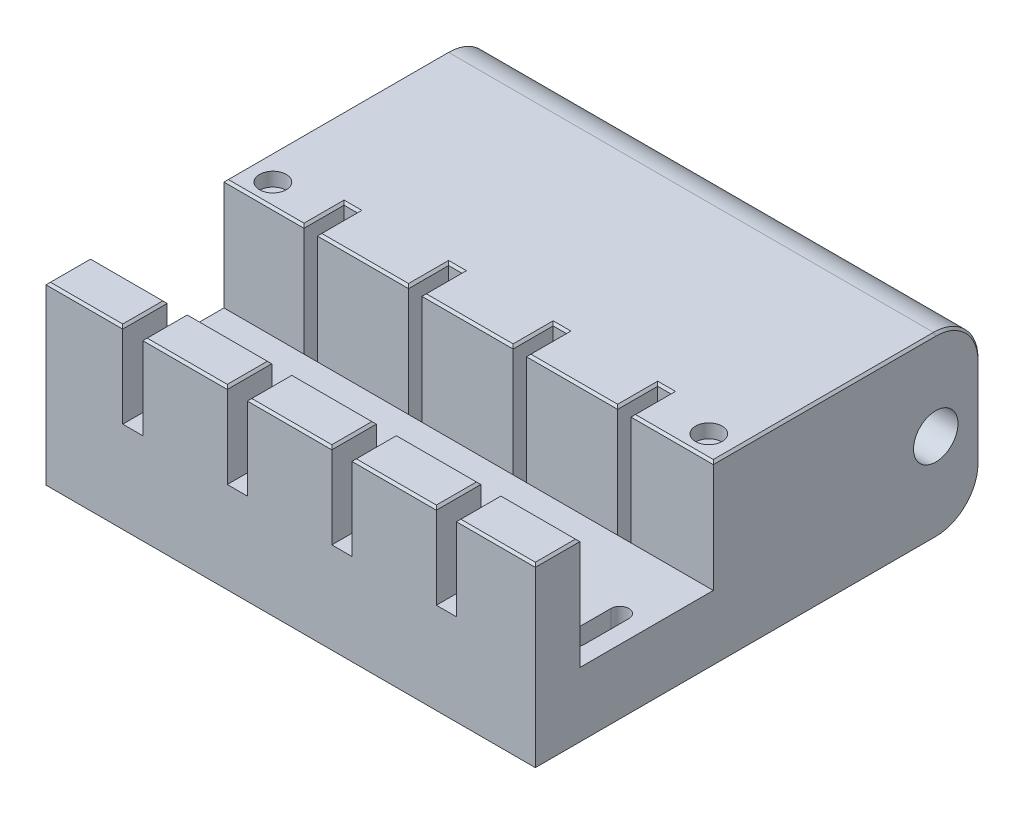
SolidWorks part; units mm, degrees
ref_plane "Front Plane" through (0, 0, 0) normal (0, 0, 1) x (1, 0, 0)
ref_plane "Top Plane" through (0, 0, 0) normal (0, 1, 0) x (1, 0, 0)
ref_plane "Right Plane" through (0, 0, 0) normal (1, 0, 0) x (0, 0, -1)
other "Configuration Table"
sketch "Sketch7" plane through (0, 0, 0) normal (0, 1, 0) x (1, 0, 0)
  line L1 (-55, 50) -> (55, 50)
  line L2 (-55, 50) -> (-55, -50)
  line L3 (-55, -50) -> (55, -50)
  line L4 (55, 50) -> (55, -50)
  line L5 (-55, 50) -> (55, -50) construction
  line L6 (-55, -50) -> (55, 50) construction
  point P0 (0, 0)
  dimension "D1" = 110
  dimension "D2" = 100
extrude "Boss-Extrude2" add sketch "Sketch7" along normal blind 40
sketch "Sketch8" plane through (0, 40, 0) normal (0, 1, 0) x (1, 0, 0)
  line L0 (0, 50) -> (0, -50) construction
  line L1 (55, 50) -> (-55, 50) construction
  line L2 (-55, -50) -> (55, -50) construction
  line L3 (-55, 50) -> (-55, -50) construction
  line L4 (-37, -1) -> (-34, -1)
  line L5 (-37, -1) -> (-37, -10)
  line L6 (-37, -10) -> (-34, -10)
  line L7 (-34, -1) -> (-34, -10)
  line L8 (-37, -1) -> (-34, -10) construction
  line L9 (-37, -10) -> (-34, -1) construction
  line L10 (-13.5, -1) -> (-13.5, -10)
  line L11 (-13.5, -1) -> (-10.5, -1)
  line L12 (-10.5, -1) -> (-10.5, -10)
  line L13 (-13.5, -10) -> (-10.5, -10)
  line L14 (10, -1) -> (10, -10)
  line L15 (10, -1) -> (13, -1)
  line L16 (13, -1) -> (13, -10)
  line L17 (10, -10) -> (13, -10)
  line L18 (33.5, -1) -> (33.5, -10)
  line L19 (33.5, -10) -> (36.5, -10)
  line L20 (36.5, -1) -> (36.5, -10)
  line L21 (33.5, -1) -> (36.5, -1)
  point P6 (-35.5, -5.5)
  dimension "D1" = 3
  dimension "D2" = 9
  dimension "D3" = 40
  dimension "D4" = 18
  dimension "D6" = 20.5
  dimension "D8" = 23.5
  dimension "D5" = 3
  dimension "D7" = 2
extrude "Cut-Extrude1" cut sketch "Sketch8" against normal through all
sketch "Sketch9" plane through (55, 0, 0) normal (1, 0, 0) x (0, 0, -1)
  line L0 (-40, 15) -> (-40, 40)
  line L2 (-50, 40) -> (50, 40) construction
  line L3 (-40, 15) -> (-10, 15)
  line L4 (-40, 40) -> (-10, 40)
  line L5 (-10, 40) -> (-10, 15)
  line L6 (-50, 40) -> (-50, 0) construction
  dimension "D1" = 25
  dimension "D2" = 10
  dimension "D4" = 30
sketch "Sketch11" plane through (0, 40, 0) normal (0, 1, 0) x (1, 0, 0)
  line L0 (-37, -10) -> (-34, -10) construction
  line L1 (-37.75, -35) -> (-33.25, -35)
  line L2 (-37.75, -35) -> (-37.75, -52)
  line L3 (-37.75, -52) -> (-33.25, -52)
  line L4 (-33.25, -35) -> (-33.25, -52)
  line L5 (-55, -50) -> (55, -50) construction
  line L6 (-14.25, -35) -> (-14.25, -52)
  line L7 (-14.25, -35) -> (-9.75, -35)
  line L8 (-9.75, -35) -> (-9.75, -52)
  line L9 (-14.25, -52) -> (-9.75, -52)
  line L10 (9.25, -35) -> (9.25, -52)
  line L11 (9.25, -35) -> (13.75, -35)
  line L12 (13.75, -35) -> (13.75, -52)
  line L13 (9.25, -52) -> (13.75, -52)
  line L14 (32.75, -35) -> (32.75, -52)
  line L15 (32.75, -35) -> (37.25, -35)
  line L16 (37.25, -35) -> (37.25, -52)
  line L17 (32.75, -52) -> (37.25, -52)
  point P6 (-35.5, -10)
  point P7 (-35.5, -35)
  dimension "D1" = 4.5
  dimension "D2" = 17
  dimension "D3" = 15
  dimension "D5" = 70.5
  dimension "D4" = 4
extrude "Cut-Extrude4" cut sketch "Sketch11" against normal blind 19
extrude "Cut-Extrude5" cut sketch "Sketch9" against normal through all contours L3 L5 L4 L0
sketch "Sketch12" plane through (55, 0, 0) normal (1, 0, 0) x (0, 0, -1)
  line L0 (50, 40) -> (50, 0) construction
  circle A0 centre (40, 20) radius 5
  point P4 (50, 20)
  dimension "D1" = 10
  dimension "D2" = 10
extrude "Cut-Extrude6" cut sketch "Sketch12" against normal through all
sketch "Sketch13" plane through (0, 21, 0) normal (0, 1, 0) x (1, 0, 0)
  line L0 (-55, -40) -> (55, -40) construction
  line L2 (-55, -40) -> (-55, -10) construction
  line L3 (55, -40) -> (55, -10) construction
  point P0 (-49, -35)
  point P1 (49, -35)
  dimension "D1" = 5
  dimension "D2" = 6
  dimension "D3" = 6
hole_wizard "Ø4.0 (4) Diameter Hole1" positions "Sketch14" profile "Sketch15" hole size "Ø4.0" standard "GB" end condition through all
sketch "Sketch14" plane through (0, 21, 0) normal (0, 1, 0) x (1, 0, 0)
  point P0 (-49, -35)
  point P3 (49, -35)
sketch "Sketch15" plane through (-49, 21, 35) normal (1, 0, 0) x (0, 0, 1)
  line L0 (0, 0) -> (0, 21)
  line L1 (0, 21) -> (2, 21)
  line L2 (2, 21) -> (2, 0)
  line L5 (2, 0) -> (0, 0)
  line L11 (0, -6.35) -> (0, 107.95) construction
  dimension "通孔孔直径" = 4
  dimension "通孔孔深度" = 21
sketch "Sketch18" plane through (0, 0, 0) normal (0, -1, 0) x (1, 0, 0)
  line L0 (-49, 35) -> (-49, 25) construction
  line L1 (-47, 35) -> (-47, 25)
  line L2 (-51, 35) -> (-51, 25)
  line L3 (0, 50) -> (0, -50) construction
  line L4 (-55, 50) -> (55, 50) construction
  line L5 (55, -50) -> (-55, -50) construction
  line L6 (49, 35) -> (49, 25) construction
  line L7 (47, 35) -> (47, 25)
  line L8 (51, 35) -> (51, 25)
  arc A0 (-47, 35) -> (-51, 35) centre (-49, 35) ccw
  arc A1 (-51, 25) -> (-47, 25) centre (-49, 25) ccw
  circle A2 centre (-49, 35) radius 2 construction
  arc A3 (47, 35) -> (51, 35) centre (49, 35) cw
  arc A4 (51, 25) -> (47, 25) centre (49, 25) cw
  point P2 (-49, 30)
  point P17 (49, 30)
  dimension "D1" = 10
extrude "Cut-Extrude8" cut sketch "Sketch18" against normal through all
sketch "Sketch19" plane through (0, 0, 0) normal (0, -1, 0) x (1, 0, 0)
  line L4 (-53, 35) -> (-53, 25)
  line L5 (-45, 25) -> (-45, 35)
  line L6 (-53, 35) -> (-53, 25)
  line L7 (-45, 25) -> (-45, 35)
  line L10 (45, 35) -> (45, 25)
  line L11 (53, 25) -> (53, 35)
  line L12 (45, 35) -> (45, 25)
  line L13 (53, 25) -> (53, 35)
  arc A4 (-45, 35) -> (-53, 35) centre (-49, 35) ccw
  arc A5 (-53, 25) -> (-45, 25) centre (-49, 25) ccw
  arc A6 (-45, 35) -> (-53, 35) centre (-49, 35) ccw
  arc A7 (-53, 25) -> (-45, 25) centre (-49, 25) ccw
  arc A10 (53, 35) -> (45, 35) centre (49, 35) ccw
  arc A11 (45, 25) -> (53, 25) centre (49, 25) ccw
  arc A12 (53, 35) -> (45, 35) centre (49, 35) ccw
  arc A13 (45, 25) -> (53, 25) centre (49, 25) ccw
  dimension "D1" = 2
  dimension "D2" = 2
extrude "Cut-Extrude9" cut sketch "Sketch19" against normal blind 5
fillet "Fillet1" radius 10 2 edges at (0, 0, -50) (0, 40, -50)
chamfer "Chamfer1" distance 0.5 angle 45 1 edges at (0, 0, 50)
chamfer "Chamfer2" distance 0.5 angle 45 27 edges at (-55, 0, 4.75) (55, 0, 4.75) (-55, 2.9289, -47.0711) (55, 2.9289, -47.0711) (-55, 20, -50) (55, 20, -50) (-55, 37.0711, -47.0711) (55, 37.0711, -47.0711) (-55, 40, -15) (-46, 40, 10) (-37, 40, 5.5) (-35.5, 40, 1) (-34, 40, 5.5) (-23.75, 40, 10) (-13.5, 40, 5.5) (-12, 40, 1) (-10.5, 40, 5.5) (-0.25, 40, 10) (10, 40, 5.5) (11.5, 40, 1) (13, 40, 5.5) (23.25, 40, 10) (33.5, 40, 5.5) (35, 40, 1) (36.5, 40, 5.5) (45.75, 40, 10) (55, 40, -15)
chamfer "Chamfer3" distance 0.5 angle 45 20 edges at (23.25, 40, 50) (13.75, 40, 45) (23.25, 40, 40) (32.75, 40, 45) (-0.25, 40, 50) (-9.75, 40, 45) (-0.25, 40, 40) (9.25, 40, 45) (-23.75, 40, 50) (-33.25, 40, 45) (-23.75, 40, 40) (-14.25, 40, 45) (-37.75, 40, 45) (-46.375, 40, 50) (-55, 40, 45) (-46.375, 40, 40) (46.125, 40, 50) (37.25, 40, 45) (46.125, 40, 40) (55, 40, 45)
sketch "Sketch20" plane through (0, 40, 0) normal (0, 1, 0) x (1, 0, 0)
  line L0 (-55, -10) -> (-55, 40) construction
  line L1 (55, 40) -> (55, -10) construction
  line L2 (-37, -10) -> (-55, -10) construction
  circle A0 centre (-49, -5) radius 3
  circle A1 centre (49, -5) radius 3
  dimension "D3" = 6
  dimension "D4" = 6
  dimension "D1" = 6
  dimension "D2" = 6
  dimension "D5" = 5
extrude "Cut-Extrude10" cut sketch "Sketch20" against normal blind 3.1
